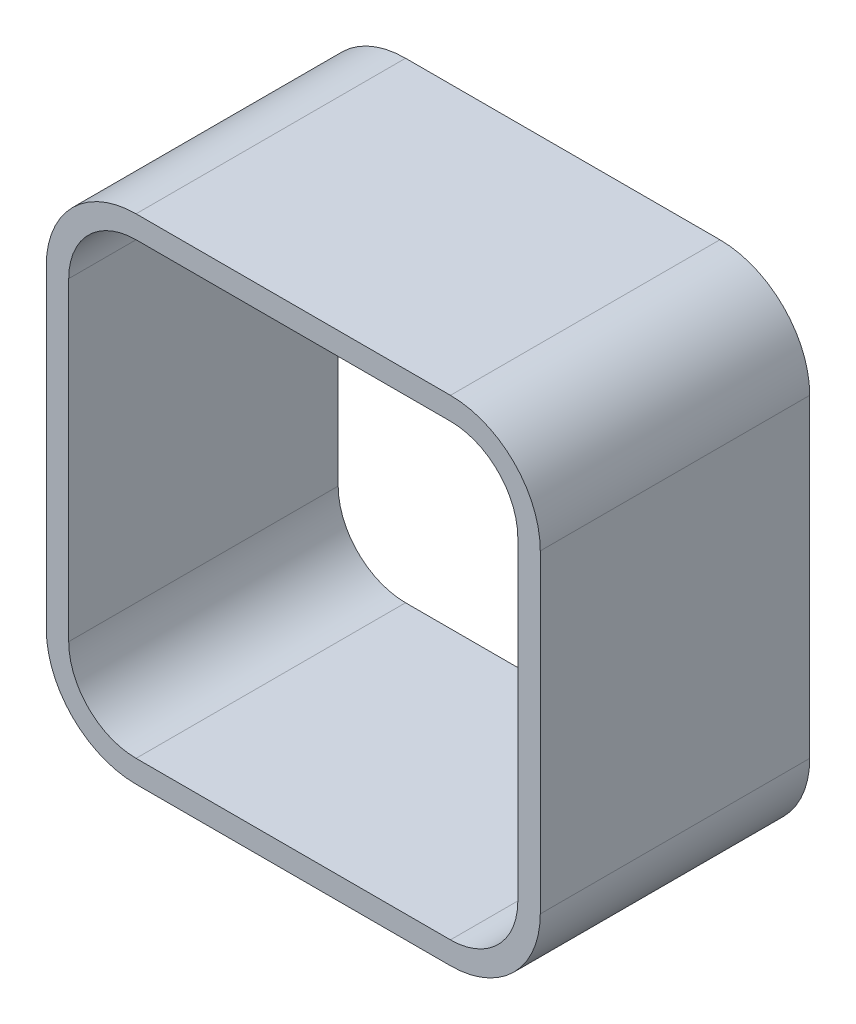
SolidWorks part; units mm, degrees
material "Q345"
ref_plane "前视基准面" through (0, 0, 0) normal (0, 0, 1) x (1, 0, 0)
ref_plane "上视基准面" through (0, 0, 0) normal (0, 1, 0) x (1, 0, 0)
ref_plane "右视基准面" through (0, 0, 0) normal (1, 0, 0) x (0, 0, -1)
sketch "草图1" plane through (0, 0, 0) normal (0, 0, 1) x (1, 0, 0)
  line L0 (-70, 110) -> (70, 110)
  line L1 (-70, 100) -> (70, 100)
  line L2 (-100, 70) -> (-100, -70)
  line L3 (-70, -100) -> (70, -100)
  line L4 (100, 70) -> (100, -70)
  line L5 (-100, 100) -> (100, -100) construction
  line L6 (-100, -100) -> (100, 100) construction
  line L7 (110, 70) -> (110, -70)
  line L8 (-70, -110) -> (70, -110)
  line L9 (-110, 70) -> (-110, -70)
  arc A0 (70, -100) -> (100, -70) centre (70, -70) ccw
  arc A1 (-70, -100) -> (-100, -70) centre (-70, -70) cw
  arc A2 (100, 70) -> (70, 100) centre (70, 70) ccw
  arc A3 (-100, 70) -> (-70, 100) centre (-70, 70) cw
  arc A4 (110, 70) -> (70, 110) centre (70, 70) ccw
  arc A5 (70, -110) -> (110, -70) centre (70, -70) ccw
  arc A6 (-70, -110) -> (-110, -70) centre (-70, -70) cw
  arc A7 (-110, 70) -> (-70, 110) centre (-70, 70) cw
  point P0 (0, 0)
  dimension "D3" = 30
  dimension "D1" = 200
  dimension "D2" = 200
  dimension "D4" = 10
extrude "凸台-拉伸1" add sketch "草图1" along normal blind 120
